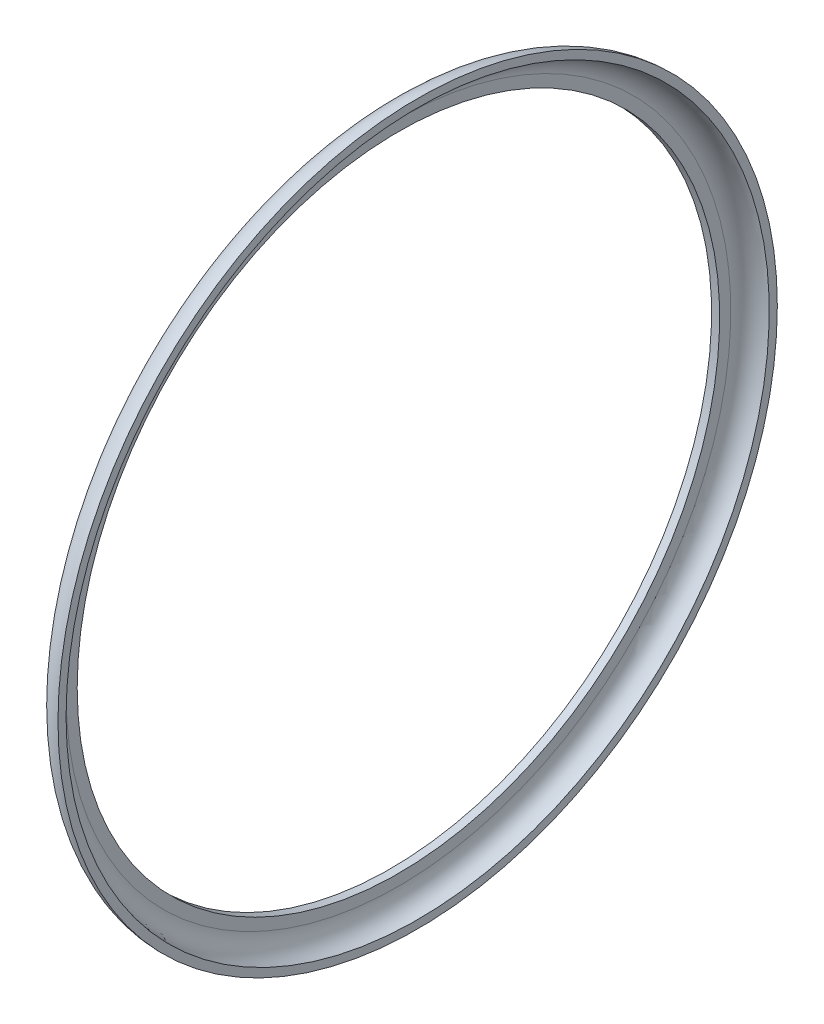
from build123d import *


with BuildPart() as part:
    # 草图1 → 旋转1 (revolve)
    with BuildSketch(Plane.XY, mode=Mode.PRIVATE) as revolve_1_sk:
        with BuildLine():
            Line((-27, 328.5), (-27, 317.5))
            Line((-27, 317.5), (-19, 317.5))
            Line((-19, 317.5), (-19, 328.5))
            ThreePointArc((-19, 328.5), (-13.435028843, 341.935028843), (0, 347.5))
            Line((0, 347.5), (0, 355.5))
            ThreePointArc((0, 355.5), (-19.091883092, 347.591883092), (-27, 328.5))
        make_face()
    revolve(revolve_1_sk.sketch.rotate(Axis((-257.766666667, 0, 0), (1, 0, 0)), 90), axis=Axis((-257.766666667, 0, 0), (1, 0, 0)))


solid = part.part
